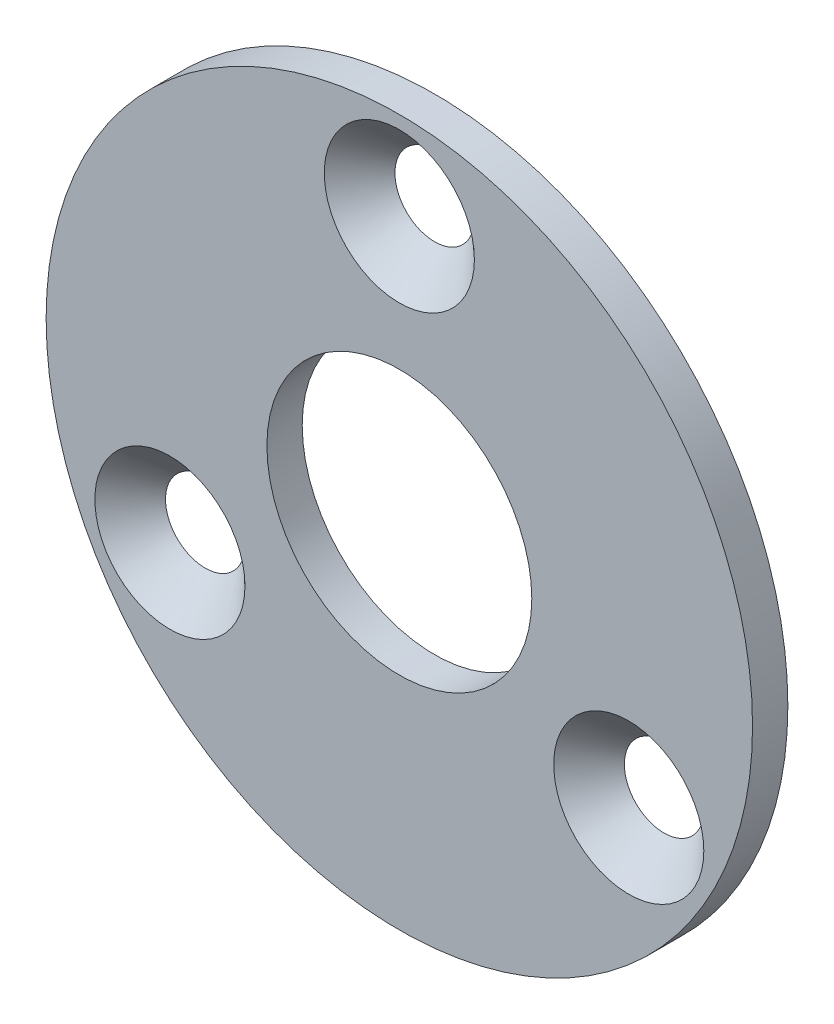
from build123d import *

# Parameters (mm, degrees)
SKETCH1_W         = 2
SKETCH1_H         = 12.5
CIRPATTERN1_COUNT = 3


with BuildPart() as part:
    # Sketch1 → Revolve1 (revolve)
    with BuildSketch(Plane(origin=(0, 0, 0), x_dir=(0, 0, -1), z_dir=(1, 0, 0)), mode=Mode.PRIVATE) as revolve1_sk:
        with Locations((1, 13.75)):
            Rectangle(SKETCH1_W, SKETCH1_H)
    revolve(revolve1_sk.sketch.rotate(Axis((0, 0, 4.366666667), (0, 0, -1)), 90), axis=Axis((0, 0, 4.366666667), (0, 0, -1)))

    # Sketch2 → Cut-Revolve1 (revolve, cut)
    with BuildSketch(Plane(origin=(0, 0, 0), x_dir=(0, 0, -1), z_dir=(1, 0, 0)), mode=Mode.PRIVATE) as cut_revolve1_sk:
        Polygon((0, 19.25), (2, 17.25), (2, 15), (0, 15), align=None)
    cut_revolve1 = revolve(cut_revolve1_sk.sketch.rotate(Axis((0, 15, 0.909195932), (0, 0, -1)), 90), axis=Axis((0, 15, 0.909195932), (0, 0, -1)), mode=Mode.SUBTRACT)

    # CirPattern1: Cut-Revolve1 ×3 about axis
    cirpattern1_axis = Axis((0, 0, 0), (0, 0, 1))
    for i in range(1, CIRPATTERN1_COUNT):
        add(cut_revolve1.rotate(cirpattern1_axis, i * 360 / CIRPATTERN1_COUNT), mode=Mode.SUBTRACT)


solid = part.part
